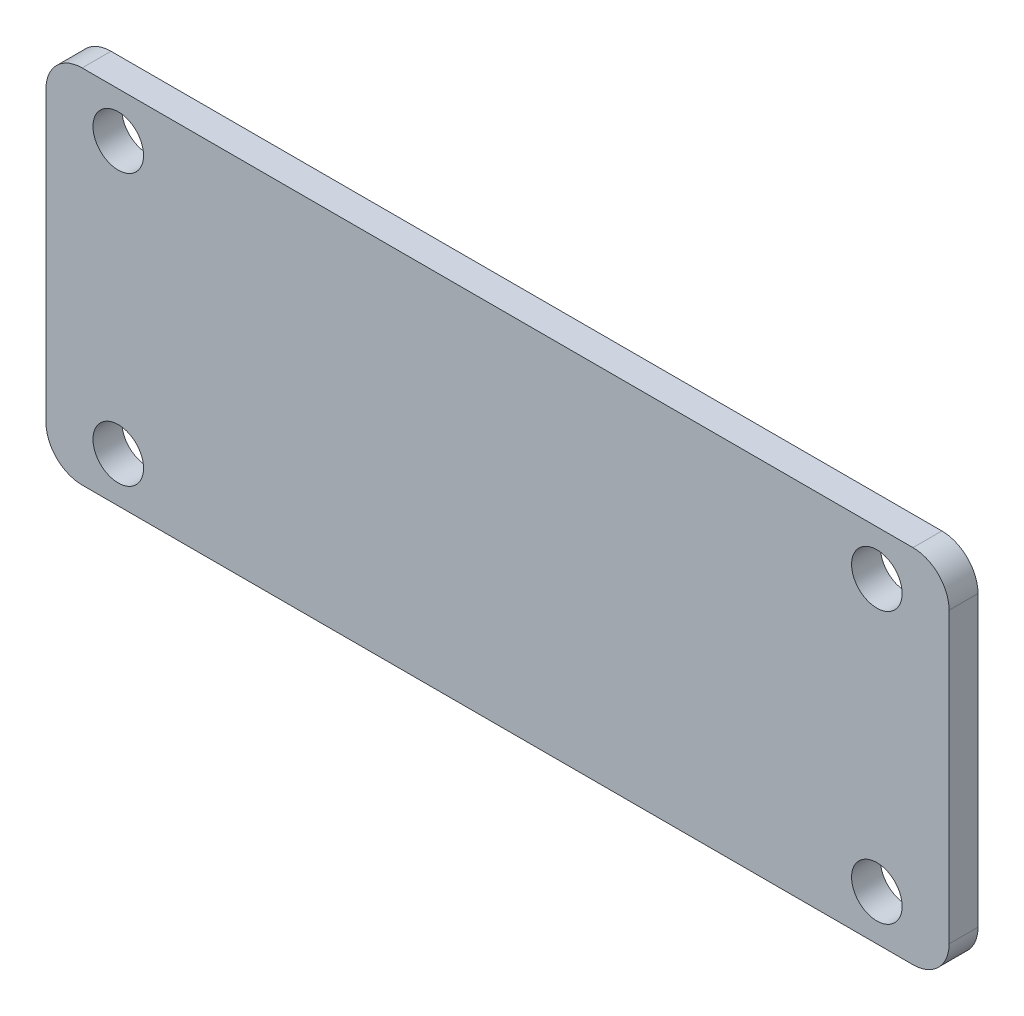
from build123d import *

# Parameters (mm, degrees)
SKETCH1_W                  = 250
SKETCH1_H                  = 100
BOSS_EXTRUDE1_DEPTH        = 4
F_14_0_14_DIAMETER_HOLE1_D = 14
FILLET1_R                  = 10


with BuildPart() as part:
    # Sketch1 → Boss-Extrude1 (new, symmetric)
    with BuildSketch(Plane.XY):
        Rectangle(SKETCH1_W, SKETCH1_H)
    extrude(amount=BOSS_EXTRUDE1_DEPTH, both=True)

    # Ø14.0 (14) Diameter Hole1 (through all)
    with Locations(Plane.XY.offset(4)):
        with Locations((-105, 37.5), (105, 37.5), (105, -37.5), (-105, -37.5)):
            Hole(F_14_0_14_DIAMETER_HOLE1_D / 2)

    # Fillet1
    fillet1_edges = [part.edges().sort_by_distance(p)[0] for p in [
        (-125, 50, 0),
        (125, 50, 0),
        (125, -50, 0),
        (-125, -50, 0),
    ]]
    fillet(fillet1_edges, radius=FILLET1_R)


solid = part.part
